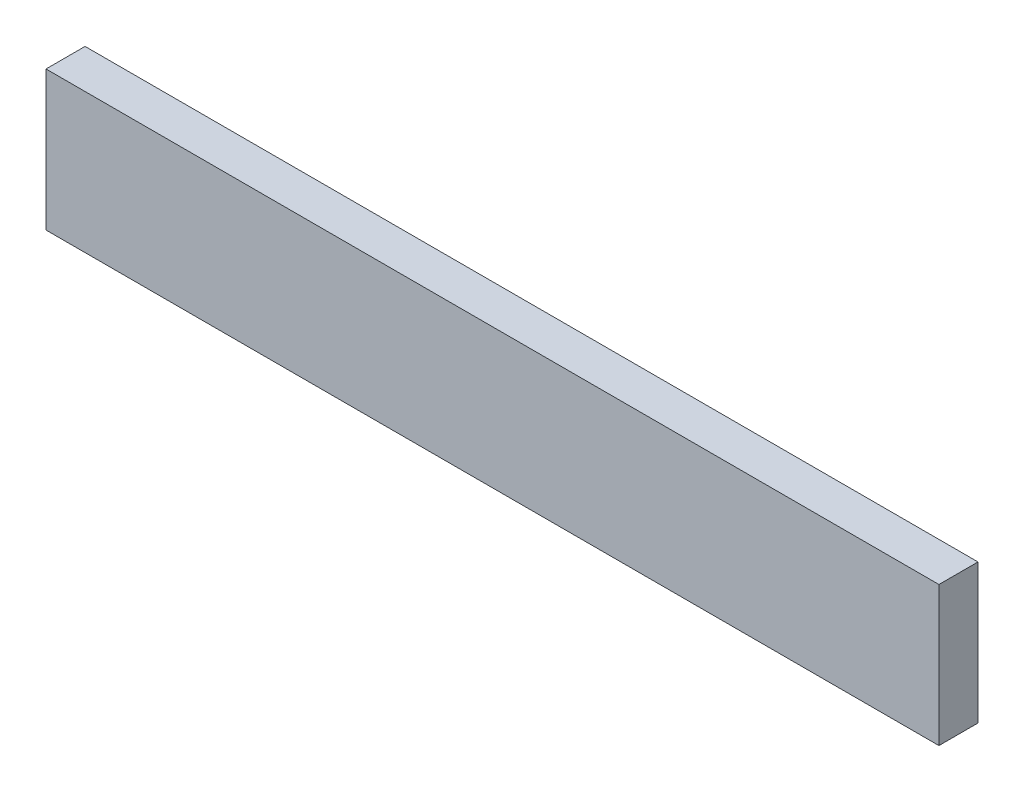
SolidWorks part; units mm, degrees
ref_plane "前视基准面" through (0, 0, 0) normal (0, 0, 1) x (1, 0, 0)
ref_plane "上视基准面" through (0, 0, 0) normal (0, 1, 0) x (1, 0, 0)
ref_plane "右视基准面" through (0, 0, 0) normal (1, 0, 0) x (0, 0, -1)
sketch "草图1" plane through (0, 0, 0) normal (0, 0, 1) x (1, 0, 0)
  line L1 (-80, -12.5) -> (80, -12.5)
  line L2 (-80, -12.5) -> (-80, 12.5)
  line L3 (-80, 12.5) -> (80, 12.5)
  line L4 (80, -12.5) -> (80, 12.5)
  line L5 (-80, -12.5) -> (80, 12.5) construction
  line L6 (-80, 12.5) -> (80, -12.5) construction
  point P0 (0, 0)
  dimension "D1" = 160
  dimension "D2" = 25
extrude "凸台-拉伸1" add sketch "草图1" along normal blind 7
